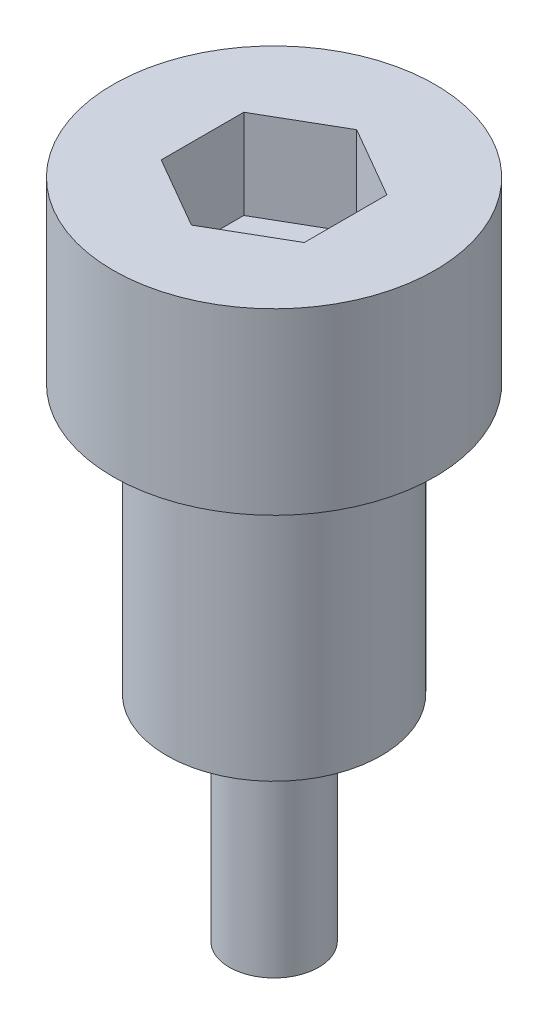
from build123d import *

# Parameters (mm, degrees)
SKETCH1_R           = 2.5
BOSS_EXTRUDE1_DEPTH = 12
SKETCH2_R           = 6
BOSS_EXTRUDE2_DEPTH = 15
SKETCH3_R           = 9
BOSS_EXTRUDE3_DEPTH = 10
CUT_EXTRUDE1_DEPTH  = 5


with BuildPart() as part:
    # Sketch1 → Boss-Extrude1 (new body)
    with BuildSketch(Plane(origin=(0, 0, 0), x_dir=(1, 0, 0), z_dir=(0, 1, 0))):
        with Locations(Location((0, 0, 0), (0, 0, 270))):
            Circle(SKETCH1_R)
    extrude(amount=BOSS_EXTRUDE1_DEPTH)

    # Sketch2 → Boss-Extrude2 (add)
    with BuildSketch(Plane(origin=(0, 12, 0), x_dir=(1, 0, 0), z_dir=(0, 1, 0))):
        with Locations(Location((0, 0, 0), (0, 0, 270))):
            Circle(SKETCH2_R)
    extrude(amount=BOSS_EXTRUDE2_DEPTH)

    # Sketch3 → Boss-Extrude3 (add)
    with BuildSketch(Plane(origin=(0, 27, 0), x_dir=(1, 0, 0), z_dir=(0, 1, 0))):
        with Locations(Location((0, 0, 0), (0, 0, 270))):
            Circle(SKETCH3_R)
    extrude(amount=BOSS_EXTRUDE3_DEPTH)

    # Sketch4 → Cut-Extrude1 (cut)
    with BuildSketch(Plane(origin=(0, 37, 0), x_dir=(1, 0, 0), z_dir=(0, 1, 0))):
        Polygon((0, 4.618802154), (-4, 2.309401077), (-4, -2.309401077), (0, -4.618802154), (4, -2.309401077), (4, 2.309401077), align=None)
    extrude(amount=-CUT_EXTRUDE1_DEPTH, mode=Mode.SUBTRACT)


solid = part.part
